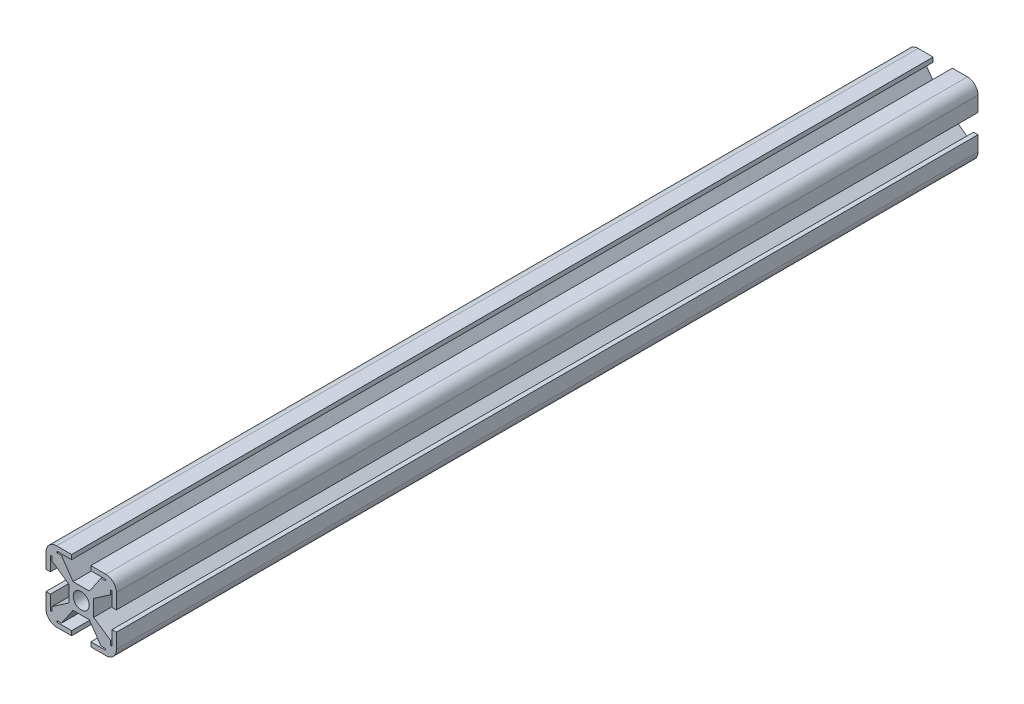
from build123d import *

# Parameters (mm, degrees)
SKETCH_1_W               = 30
SKETCH_1_H               = 30
EXTRUDE_1_DEPTH          = 183.5
FILLET_1_R               = 4.5
SKETCH_2_W               = 8.2
SKETCH_2_H               = 0.3
SKETCH_2_H_2             = 1.9
SKETCH_2_R               = 3.4
CUT_EXTRUDE_1_DEPTH      = 368.612567794
PATTERN_CIRCULAR_1_COUNT = 4


with BuildPart() as part:
    # 草图1 → 凸台-拉伸1 (new, symmetric)
    with BuildSketch(Plane.XY):
        Rectangle(SKETCH_1_W, SKETCH_1_H)
    extrude(amount=EXTRUDE_1_DEPTH, both=True)

    # 圆角1
    fillet_1_edges = [part.edges().sort_by_distance(p)[0] for p in [
        (-15, 15, 0),
        (15, 15, 0),
        (15, -15, 0),
        (-15, -15, 0),
    ]]
    fillet(fillet_1_edges, radius=FILLET_1_R)

    # 草图2 → 切除-拉伸1 (cut, through all)
    with BuildSketch(Plane.XY.offset(183.5)):
        with Locations((0, 12.95)):
            Rectangle(SKETCH_2_W, SKETCH_2_H)
        with Locations((0, 14.05)):
            Rectangle(SKETCH_2_W, SKETCH_2_H_2)
        Polygon((10.25, 13.1), (4.1, 13.1), (4.1, 12.8), (-4.1, 12.8), (-4.1, 13.1), (-10.25, 13.1), (-10.25, 12.5), (-8.429704265, 12.5), (8.429704265, 12.5), (10.25, 12.5), align=None)
        Polygon((3.479704265, 5.3), (8.429704265, 12.5), (-8.429704265, 12.5), (-3.479704265, 5.3), align=None)
        Circle(SKETCH_2_R)
    cut_extrude_1 = extrude(amount=-CUT_EXTRUDE_1_DEPTH, mode=Mode.SUBTRACT)

    # 阵列(圆周)1: 切除-拉伸1 ×4 about axis
    pattern_circular_1_axis = Axis((0, 0, 0), (0, 0, 1))
    for i in range(1, PATTERN_CIRCULAR_1_COUNT):
        add(cut_extrude_1.rotate(pattern_circular_1_axis, i * 360 / PATTERN_CIRCULAR_1_COUNT), mode=Mode.SUBTRACT)


solid = part.part
